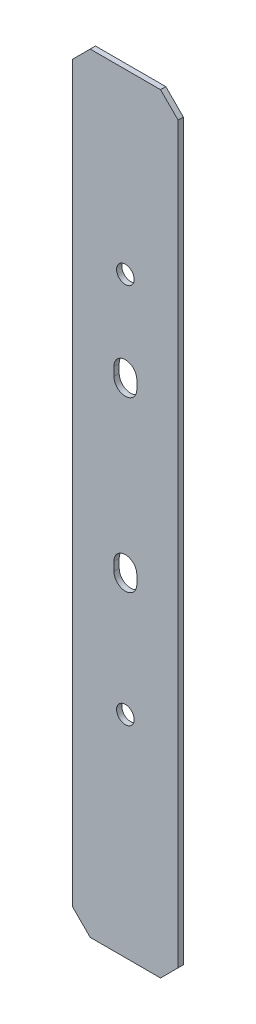
from build123d import *

# Parameters (mm, degrees)
SKETCH_1_W          = 60
SKETCH_1_H          = 437.5
EXTRUDE_1_DEPTH     = 3
CHAMFER_1_SIZE      = 10
SKETCH_2_R          = 5
CUT_EXTRUDE_1_DEPTH = 10


with BuildPart() as part:
    # 草图1 → 凸台-拉伸1 (new body)
    with BuildSketch(Plane.XY):
        with Locations((0, -18.75)):
            Rectangle(SKETCH_1_W, SKETCH_1_H)
    extrude(amount=EXTRUDE_1_DEPTH)

    # 倒角1
    chamfer_1_edges = [part.edges().sort_by_distance(p)[0] for p in [
        (30, -237.5, 1.5),
        (-30, -237.5, 1.5),
        (-30, 200, 1.5),
        (30, 200, 1.5),
    ]]
    chamfer(chamfer_1_edges, length=CHAMFER_1_SIZE)

    # 草图2 → 切除-拉伸1 (cut)
    with BuildSketch(Plane.XY.offset(3)):
        with Locations((0, 99)):
            Circle(SKETCH_2_R)
        with Locations((0, -117.75)):
            Circle(SKETCH_2_R)
        with BuildLine():
            Line((6.5, 50.5), (6.5, 45.5))
            ThreePointArc((6.5, 45.5), (0, 39), (-6.5, 45.5))
            Line((-6.5, 45.5), (-6.5, 50.5))
            ThreePointArc((-6.5, 50.5), (0, 57), (6.5, 50.5))
        make_face()
        with BuildLine():
            Line((6.5, -45.5), (6.5, -50.5))
            ThreePointArc((6.5, -50.5), (0, -57), (-6.5, -50.5))
            Line((-6.5, -50.5), (-6.5, -45.5))
            ThreePointArc((-6.5, -45.5), (0, -39), (6.5, -45.5))
        make_face()
    extrude(amount=-CUT_EXTRUDE_1_DEPTH, mode=Mode.SUBTRACT)


solid = part.part
